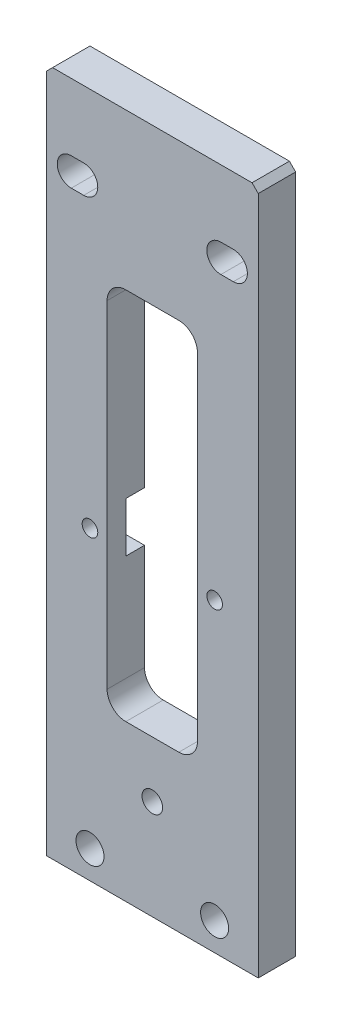
SolidWorks part; units mm, degrees
ref_plane "Front Plane" through (0, 0, 0) normal (0, 0, 1) x (1, 0, 0)
ref_plane "Top Plane" through (0, 0, 0) normal (0, 1, 0) x (1, 0, 0)
ref_plane "Right Plane" through (0, 0, 0) normal (1, 0, 0) x (0, 0, -1)
sketch "Sketch1" plane through (0, 0, 0) normal (0, 0, 1) x (1, 0, 0)
  line L1 (-17, 55) -> (17, 55)
  line L2 (-17, 55) -> (-17, -55)
  line L3 (-17, -55) -> (17, -55)
  line L4 (17, 55) -> (17, -55)
  line L5 (-17, 55) -> (17, -55) construction
  line L6 (-17, -55) -> (17, 55) construction
  point P0 (0, 0)
  dimension "D1" = 34
  dimension "D2" = 110
extrude "Boss-Extrude1" add sketch "Sketch1" along normal blind 6
chamfer "Chamfer1" distance 1 angle 45 2 edges at (17, 55, 3) (-17, 55, 3)
hole_wizard "Ø4.5 (4.5) Diameter Hole1" positions "Sketch3" profile "Sketch2" hole size "Ø4.5" standard "Gb" end condition through all
sketch "Sketch3" plane through (0, 0, 0) normal (0, 0, -1) x (-1, 0, 0)
  line L0 (0, 0) -> (0, -55) construction
  line L1 (17, -55) -> (-17, -55) construction
  point P0 (-10, -50.5)
  point P3 (10, -50.5)
  dimension "D1" = 20
  dimension "D2" = 4.5
sketch "Sketch2" plane through (10, -50.5, 0) normal (1, 0, 0) x (0, 1, 0)
  line L0 (0, 0) -> (0, 6)
  line L1 (0, 6) -> (2.25, 6)
  line L2 (2.25, 6) -> (2.25, 0)
  line L5 (2.25, 0) -> (0, 0)
  line L11 (0, -6.35) -> (0, 107.95) construction
  dimension "通孔孔直径" = 4.5
  dimension "通孔孔深度" = 6
sketch "Sketch4" plane through (0, 0, 0) normal (0, 0, -1) x (-1, 0, 0)
  line L0 (-13, 42) -> (-11, 42) construction
  line L1 (-13, 44.25) -> (-11, 44.25)
  line L2 (-13, 39.75) -> (-11, 39.75)
  line L3 (11, 42) -> (13, 42) construction
  line L4 (11, 44.25) -> (13, 44.25)
  line L5 (11, 39.75) -> (13, 39.75)
  line L6 (0, 0) -> (0, 72.2166) construction
  line L8 (17, -55) -> (-17, -55) construction
  arc A0 (-13, 44.25) -> (-13, 39.75) centre (-13, 42) ccw
  arc A1 (-11, 39.75) -> (-11, 44.25) centre (-11, 42) ccw
  arc A2 (11, 44.25) -> (11, 39.75) centre (11, 42) ccw
  arc A3 (13, 39.75) -> (13, 44.25) centre (13, 42) ccw
  point P2 (-12, 42)
  point P7 (12, 42)
  dimension "D1" = 4.5
  dimension "D2" = 2
  dimension "D3" = 24
  dimension "D4" = 97
extrude "Cut-Extrude1" cut sketch "Sketch4" against normal through all
sketch "Sketch12" plane through (0, 0, 0) normal (0, 0, -1) x (-1, 0, 0)
  line L1 (-7.25, 30) -> (7.25, 30)
  line L2 (-7.25, 30) -> (-7.25, -30)
  line L3 (-7.25, -30) -> (7.25, -30)
  line L4 (7.25, 30) -> (7.25, -30)
  line L5 (-7.25, 30) -> (7.25, -30) construction
  line L6 (-7.25, -30) -> (7.25, 30) construction
  point P0 (0, 0)
  dimension "D1" = 14.5
  dimension "D2" = 60
extrude "Cut-Extrude2" cut sketch "Sketch12" against normal through all
sketch "Sketch13" plane through (0, 0, 0) normal (0, 0, -1) x (-1, 0, 0)
  line L1 (-13.5, -2) -> (13.5, -2)
  line L2 (-13.5, -2) -> (-13.5, -10)
  line L3 (-13.5, -10) -> (13.5, -10)
  line L4 (13.5, -2) -> (13.5, -10)
  line L5 (-13.5, -2) -> (13.5, -10) construction
  line L6 (-13.5, -10) -> (13.5, -2) construction
  line L7 (-7.25, -30) -> (7.25, -30) construction
  point P0 (0, -6)
  dimension "D1" = 27
  dimension "D2" = 8
  dimension "D3" = 20
extrude "Cut-Extrude3" cut sketch "Sketch13" against normal blind 3
fillet "Fillet1" radius 3 4 edges at (-7.25, -30, 3) (7.25, -30, 3) (7.25, 30, 3) (-7.25, 30, 3)
sketch "Sketch14" plane through (0, 0, 0) normal (0, 0, -1) x (-1, 0, 0)
  circle A0 centre (-13.5, -2) radius 1
  circle A1 centre (-13.5, -10) radius 1
  circle A2 centre (13.5, -10) radius 1
  circle A3 centre (13.5, -2) radius 1
  dimension "D1" = 2
extrude "Cut-Extrude4" cut sketch "Sketch14" against normal up to surface (3 mm away) up to face at (10.375, -6, 3)
hole_wizard "M3 Tapped Hole1" positions "Sketch16" profile "Sketch15" tap size "M3" standard "Gb" end condition through all
sketch "Sketch16" plane through (0, 0, 0) normal (0, 0, -1) x (-1, 0, 0)
  line L0 (0, 0) -> (0, 11.5924) construction
  line L2 (7.25, -10) -> (12.5, -10) construction
  point P0 (-10, -6)
  point P2 (10, -6)
  dimension "D1" = 20
  dimension "D2" = 4
sketch "Sketch15" plane through (10, -6, 0) normal (1, 0, 0) x (0, 1, 0)
  line L0 (0, 0) -> (0, 6)
  line L1 (0, 6) -> (1.25, 6)
  line L2 (1.25, 6) -> (1.25, 0)
  line L5 (1.25, 0) -> (0, 0)
  line L11 (0, -6.35) -> (0, 107.95) construction
  dimension "通孔螺纹孔钻头直径" = 2.5
  dimension "通孔螺纹孔钻头深度" = 6
cosmetic thread "Cosmetic Thread1" parameters "D2"=3
cosmetic thread "Cosmetic Thread2" parameters "D2"=3
hole_wizard "M4 Tapped Hole1" positions "Sketch18" profile "Sketch17" tap size "M4" standard "Gb" end condition through all
sketch "Sketch18" plane through (0, 0, 6) normal (0, 0, 1) x (1, 0, 0)
  line L0 (-17, -55) -> (17, -55) construction
  point P0 (0, -39)
  dimension "D1" = 16
sketch "Sketch17" plane through (0, -39, 6) normal (1, 0, 0) x (0, -1, 0)
  line L0 (0, 0) -> (0, 6)
  line L1 (0, 6) -> (1.65, 6)
  line L2 (1.65, 6) -> (1.65, 0)
  line L5 (1.65, 0) -> (0, 0)
  line L11 (0, -6.35) -> (0, 107.95) construction
  dimension "通孔螺纹孔钻头直径" = 3.3
  dimension "通孔螺纹孔钻头深度" = 6
cosmetic thread "Cosmetic Thread3" parameters "D2"=4
